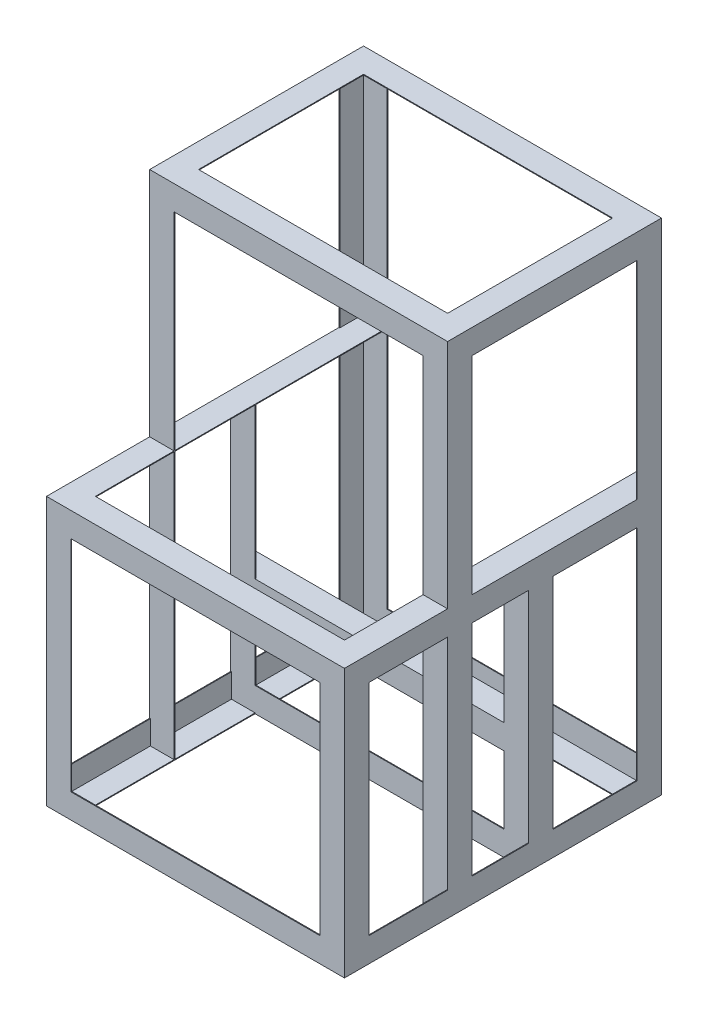
from build123d import *

# Parameters (mm, degrees)
BOSS_EXTRUDE1_DEPTH   = 1308
BOSS_EXTRUDE2_DEPTH   = 828
BOSS_EXTRUDE3_DEPTH   = 700
BOSS_EXTRUDE4_DEPTH   = 828
BOSS_EXTRUDE5_DEPTH   = 558
BOSS_EXTRUDE6_REACH   = 1517.417
BOSS_EXTRUDE8_DEPTH   = 388
MIRROR4_COPY_1_DEPTH  = 1308
MIRROR4_COPY_2_DEPTH  = 828
MIRROR4_COPY_3_DEPTH  = 700
MIRROR4_COPY_4_DEPTH  = 828
MIRROR4_COPY_5_DEPTH  = 558
MIRROR4_COPY_6_REACH  = 1517.417
MIRROR4_COPY_7_DEPTH  = 388
MIRROR4_COPY_8_DEPTH  = 1308
MIRROR4_COPY_9_DEPTH  = 828
MIRROR4_COPY_10_DEPTH = 700
MIRROR4_COPY_11_DEPTH = 828
MIRROR4_COPY_12_DEPTH = 558
MIRROR4_COPY_13_REACH = 1517.417
MIRROR4_COPY_14_DEPTH = 388
BOSS_EXTRUDE9_REACH   = 1706.705
BOSS_EXTRUDE10_DEPTH  = 778
BOSS_EXTRUDE11_START  = -778
BOSS_EXTRUDE11_DEPTH  = 776


with BuildPart() as part:
    # Sketch1 → Boss-Extrude1 (new body)
    with BuildSketch(Plane(origin=(0, 0, 0), x_dir=(1, 0, 0), z_dir=(0, 1, 0))):
        Polygon((0, 0), (0, 64), (64, 64), (64, 62), (2, 62), (2, 0), align=None)
    boss_extrude1 = extrude(amount=BOSS_EXTRUDE1_DEPTH)

    # Sketch2 → Boss-Extrude2 (add)
    with BuildSketch(Plane.XY.offset(-62)):
        Polygon((64, 0), (0, 0), (0, 64), (2, 64), (2, 2), (64, 2), align=None)
    boss_extrude2 = extrude(amount=BOSS_EXTRUDE2_DEPTH)

    # Sketch3 → Boss-Extrude3 (add)
    with BuildSketch(Plane(origin=(0, 2, 0), x_dir=(1, 0, 0), z_dir=(0, 1, 0))):
        Polygon((64, -766), (0, -766), (0, -702), (2, -702), (2, -764), (64, -764), align=None)
    boss_extrude3 = extrude(amount=BOSS_EXTRUDE3_DEPTH)

    # Sketch4 → Boss-Extrude4 (add)
    with BuildSketch(Plane(origin=(0, 0, 764), x_dir=(-1, 0, 0), z_dir=(0, 0, -1))):
        Polygon((-64, 702), (0, 702), (0, 638), (-2, 638), (-2, 700), (-64, 700), align=None)
    boss_extrude4 = extrude(amount=BOSS_EXTRUDE4_DEPTH)

    # Sketch5 → Boss-Extrude5 (add)
    with BuildSketch(Plane.XY.offset(-62)):
        Polygon((64, 1308), (0, 1308), (0, 1244), (2, 1244), (2, 1306), (64, 1306), align=None)
    boss_extrude5 = extrude(amount=BOSS_EXTRUDE5_DEPTH)

    # Boss-Extrude6: up to this face of the body (flat: up to its plane)
    boss_extrude6_end = Plane(part.part.faces().sort_by_distance((33, 2, 351))[0])
    # Sketch6 → Boss-Extrude6 (add, up to the picked face)
    with BuildSketch(Plane.XZ.offset(-1306), mode=Mode.PRIVATE) as boss_extrude6_sk1:
        Polygon((64, 496), (0, 496), (0, 432), (2, 432), (2, 494), (64, 494), align=None)
    boss_extrude6_tool1 = split(extrude(boss_extrude6_sk1.sketch, amount=BOSS_EXTRUDE6_REACH, mode=Mode.PRIVATE), bisect_by=boss_extrude6_end, keep=Keep.BOTH, mode=Mode.PRIVATE)
    boss_extrude6 = boss_extrude6_tool1.solids().sort_by(Axis((32, 1306, 495.094903), (0, -1, 0)))[0]
    add(boss_extrude6)

    # Sketch7 → Boss-Extrude8 (add)
    with BuildSketch(Plane(origin=(2, 0, 0), x_dir=(0, 0, -1), z_dir=(1, 0, 0))):
        Polygon((-496, 1308), (-432, 1308), (-432, 1306), (-494, 1306), (-494, 1244), (-496, 1244), align=None)
        Polygon((64, 1308), (0, 1308), (0, 1306), (62, 1306), (62, 1244), (64, 1244), align=None)
        Polygon((64, 0), (64, 64), (62, 64), (62, 2), (0, 2), (0, 0), align=None)
        Polygon((-766, 0), (-766, 64), (-763.755809275, 64), (-764, 2), (-702, 2), (-702, 0), align=None)
        Polygon((-766, 702), (-702, 702), (-702, 700), (-764, 700), (-764, 638), (-766, 638), align=None)
    boss_extrude8 = extrude(amount=BOSS_EXTRUDE8_DEPTH)

    # Mirror4 copy 1 sketch → Mirror4 copy 1 (add)
    with BuildSketch(Plane(origin=(0, 0, 0), x_dir=(1, 0, 0), z_dir=(0, 1, 0))):
        Polygon((0, 0), (0, 64), (64, 64), (64, 62), (2, 62), (2, 0), align=None)
    extrude(amount=MIRROR4_COPY_1_DEPTH)

    # Mirror4 copy 2 sketch → Mirror4 copy 2 (add)
    with BuildSketch(Plane.XY.offset(-62)):
        Polygon((64, 0), (0, 0), (0, 64), (2, 64), (2, 2), (64, 2), align=None)
    extrude(amount=MIRROR4_COPY_2_DEPTH)

    # Mirror4 copy 3 sketch → Mirror4 copy 3 (add)
    with BuildSketch(Plane(origin=(0, 2, 0), x_dir=(1, 0, 0), z_dir=(0, 1, 0))):
        Polygon((64, -766), (0, -766), (0, -702), (2, -702), (2, -764), (64, -764), align=None)
    extrude(amount=MIRROR4_COPY_3_DEPTH)

    # Mirror4 copy 4 sketch → Mirror4 copy 4 (add)
    with BuildSketch(Plane(origin=(0, 0, 764), x_dir=(-1, 0, 0), z_dir=(0, 0, -1))):
        Polygon((-64, 702), (0, 702), (0, 638), (-2, 638), (-2, 700), (-64, 700), align=None)
    extrude(amount=MIRROR4_COPY_4_DEPTH)

    # Mirror4 copy 5 sketch → Mirror4 copy 5 (add)
    with BuildSketch(Plane.XY.offset(-62)):
        Polygon((64, 1308), (0, 1308), (0, 1244), (2, 1244), (2, 1306), (64, 1306), align=None)
    extrude(amount=MIRROR4_COPY_5_DEPTH)

    # Mirror4 copy 6: up to this face of the body (flat: up to its plane)
    mirror4_copy_6_end = Plane(part.part.faces().sort_by_distance((33, 2, 351))[0])
    # Mirror4 copy 6 sketch → Mirror4 copy 6 (add, up to the picked face)
    with BuildSketch(Plane.XZ.offset(-1306), mode=Mode.PRIVATE) as mirror4_copy_6_sk1:
        Polygon((64, 496), (0, 496), (0, 432), (2, 432), (2, 494), (64, 494), align=None)
    mirror4_copy_6_tool1 = split(extrude(mirror4_copy_6_sk1.sketch, amount=MIRROR4_COPY_6_REACH, mode=Mode.PRIVATE), bisect_by=mirror4_copy_6_end, keep=Keep.BOTH, mode=Mode.PRIVATE)
    add(mirror4_copy_6_tool1.solids().sort_by(Axis((32, 1306, 495.094903), (0, -1, 0)))[0])



with BuildPart() as mirror3_1:
    # Mirror3: Boss-Extrude1, Boss-Extrude2, Boss-Extrude3, Boss-Extrude4, Boss-Extrude5, Boss-Extrude6, Boss-Extrude8 across plane
    add(boss_extrude1.mirror(Plane(origin=(390, 0, 0), x_dir=(0, 0, 1), z_dir=(1, 0, 0))))
    add(boss_extrude2.mirror(Plane(origin=(390, 0, 0), x_dir=(0, 0, 1), z_dir=(1, 0, 0))))
    add(boss_extrude3.mirror(Plane(origin=(390, 0, 0), x_dir=(0, 0, 1), z_dir=(1, 0, 0))))
    add(boss_extrude4.mirror(Plane(origin=(390, 0, 0), x_dir=(0, 0, 1), z_dir=(1, 0, 0))))
    add(boss_extrude5.mirror(Plane(origin=(390, 0, 0), x_dir=(0, 0, 1), z_dir=(1, 0, 0))))
    add(boss_extrude6.mirror(Plane(origin=(390, 0, 0), x_dir=(0, 0, 1), z_dir=(1, 0, 0))))
    add(boss_extrude8.mirror(Plane(origin=(390, 0, 0), x_dir=(0, 0, 1), z_dir=(1, 0, 0))))


with BuildPart() as part_1:
    add(part.part)

    add(mirror3_1.part)  # Mirror4 copy 7 merges Mirror3_1
    # Mirror4 copy 7 sketch → Mirror4 copy 7 (add)
    with BuildSketch(Plane(origin=(2, 0, 0), x_dir=(0, 0, -1), z_dir=(1, 0, 0))):
        Polygon((-496, 1308), (-432, 1308), (-432, 1306), (-494, 1306), (-494, 1244), (-496, 1244), align=None)
        Polygon((64, 1308), (0, 1308), (0, 1306), (62, 1306), (62, 1244), (64, 1244), align=None)
        Polygon((64, 0), (64, 64), (62, 64), (62, 2), (0, 2), (0, 0), align=None)
        Polygon((-766, 0), (-766, 64), (-763.755809275, 64), (-764, 2), (-702, 2), (-702, 0), align=None)
        Polygon((-766, 702), (-702, 702), (-702, 700), (-764, 700), (-764, 638), (-766, 638), align=None)
    extrude(amount=MIRROR4_COPY_7_DEPTH)

    # Mirror4 copy 8 sketch → Mirror4 copy 8 (add)
    with BuildSketch(Plane(origin=(780, 0, 0), x_dir=(-1, 0, 0), z_dir=(0, 1, 0))):
        Polygon((0, 0), (0, -64), (64, -64), (64, -62), (2, -62), (2, 0), align=None)
    extrude(amount=MIRROR4_COPY_8_DEPTH)

    # Mirror4 copy 9 sketch → Mirror4 copy 9 (add)
    with BuildSketch(Plane(origin=(780, 0, -62), x_dir=(-1, 0, 0), z_dir=(0, 0, 1))):
        Polygon((64, 0), (0, 0), (0, -64), (2, -64), (2, -2), (64, -2), align=None)
    extrude(amount=MIRROR4_COPY_9_DEPTH)

    # Mirror4 copy 10 sketch → Mirror4 copy 10 (add)
    with BuildSketch(Plane(origin=(780, 2, 0), x_dir=(-1, 0, 0), z_dir=(0, 1, 0))):
        Polygon((64, 766), (0, 766), (0, 702), (2, 702), (2, 764), (64, 764), align=None)
    extrude(amount=MIRROR4_COPY_10_DEPTH)

    # Mirror4 copy 11 sketch → Mirror4 copy 11 (add)
    with BuildSketch(Plane(origin=(780, 0, 764), x_dir=(1, 0, 0), z_dir=(0, 0, -1))):
        Polygon((-64, -702), (0, -702), (0, -638), (-2, -638), (-2, -700), (-64, -700), align=None)
    extrude(amount=MIRROR4_COPY_11_DEPTH)

    # Mirror4 copy 12 sketch → Mirror4 copy 12 (add)
    with BuildSketch(Plane(origin=(780, 0, -62), x_dir=(-1, 0, 0), z_dir=(0, 0, 1))):
        Polygon((64, -1308), (0, -1308), (0, -1244), (2, -1244), (2, -1306), (64, -1306), align=None)
    extrude(amount=MIRROR4_COPY_12_DEPTH)

    # Mirror4 copy 13: up to this face of the body (flat: up to its plane)
    mirror4_copy_13_end = Plane(part_1.part.faces().sort_by_distance((747, 2, 351))[0])
    # Mirror4 copy 13 sketch → Mirror4 copy 13 (add, up to the picked face)
    with BuildSketch(Plane(origin=(780, 1306, 0), x_dir=(-1, 0, 0), z_dir=(0, -1, 0)), mode=Mode.PRIVATE) as mirror4_copy_13_sk1:
        Polygon((64, -496), (0, -496), (0, -432), (2, -432), (2, -494), (64, -494), align=None)
    mirror4_copy_13_tool1 = split(extrude(mirror4_copy_13_sk1.sketch, amount=MIRROR4_COPY_13_REACH, mode=Mode.PRIVATE), bisect_by=mirror4_copy_13_end, keep=Keep.BOTH, mode=Mode.PRIVATE)
    add(mirror4_copy_13_tool1.solids().sort_by(Axis((748, 1306, 495.094903), (0, -1, 0)))[0])

    # Mirror4 copy 14 sketch → Mirror4 copy 14 (add)
    with BuildSketch(Plane(origin=(778, 0, 0), x_dir=(0, 0, -1), z_dir=(-1, 0, 0))):
        Polygon((-496, -1308), (-432, -1308), (-432, -1306), (-494, -1306), (-494, -1244), (-496, -1244), align=None)
        Polygon((64, -1308), (0, -1308), (0, -1306), (62, -1306), (62, -1244), (64, -1244), align=None)
        Polygon((64, 0), (64, -64), (62, -64), (62, -2), (0, -2), (0, 0), align=None)
        Polygon((-766, 0), (-766, -64), (-763.755809275, -64), (-764, -2), (-702, -2), (-702, 0), align=None)
        Polygon((-766, -702), (-702, -702), (-702, -700), (-764, -700), (-764, -638), (-766, -638), align=None)
    extrude(amount=MIRROR4_COPY_14_DEPTH)

    # Boss-Extrude9: up to this face of the body (flat: up to its plane)
    boss_extrude9_end = Plane(part_1.part.faces().sort_by_distance((33, 700, 216))[0])
    # Sketch8 → Boss-Extrude9 (add, up to the picked face)
    with BuildSketch(Plane.XZ, mode=Mode.PRIVATE) as boss_extrude9_sk1:
        Polygon((0, 283.816221782), (64, 283.816221782), (64, 281.816221782), (2, 281.816221782), (2, 219.816221782), (0, 219.816221782), align=None)
    boss_extrude9_tool1 = split(extrude(boss_extrude9_sk1.sketch, amount=-BOSS_EXTRUDE9_REACH, mode=Mode.PRIVATE), bisect_by=boss_extrude9_end, keep=Keep.BOTH, mode=Mode.PRIVATE)
    boss_extrude9 = boss_extrude9_tool1.solids().sort_by(Axis((32, 0, 282.911125), (0, 1, 0)))[0]
    add(boss_extrude9)

    # Mirror5: Boss-Extrude9 across plane
    add(boss_extrude9.mirror(Plane(origin=(390, 0, 0), x_dir=(0, 0, 1), z_dir=(1, 0, 0))))

    # Sketch9 → Boss-Extrude10 (add)
    with BuildSketch(Plane.ZY):
        Polygon((283.816221782, 64), (283.816221782, 0), (219.816221782, 0), (219.816221782, 2), (281.816221782, 2), (281.816221782, 64), align=None)
    extrude(amount=-BOSS_EXTRUDE10_DEPTH)

    # Sketch10 → Boss-Extrude11 (add)
    with BuildSketch(Plane.ZY.offset(BOSS_EXTRUDE11_START)):
        Polygon((219.816221782, 305.547407483), (283.816221782, 305.547407483), (283.816221782, 241.547407483), (281.816221782, 241.547407483), (281.816221782, 303.547407483), (219.816221782, 303.547407483), align=None)
    extrude(amount=BOSS_EXTRUDE11_DEPTH)


solid = part_1.part
